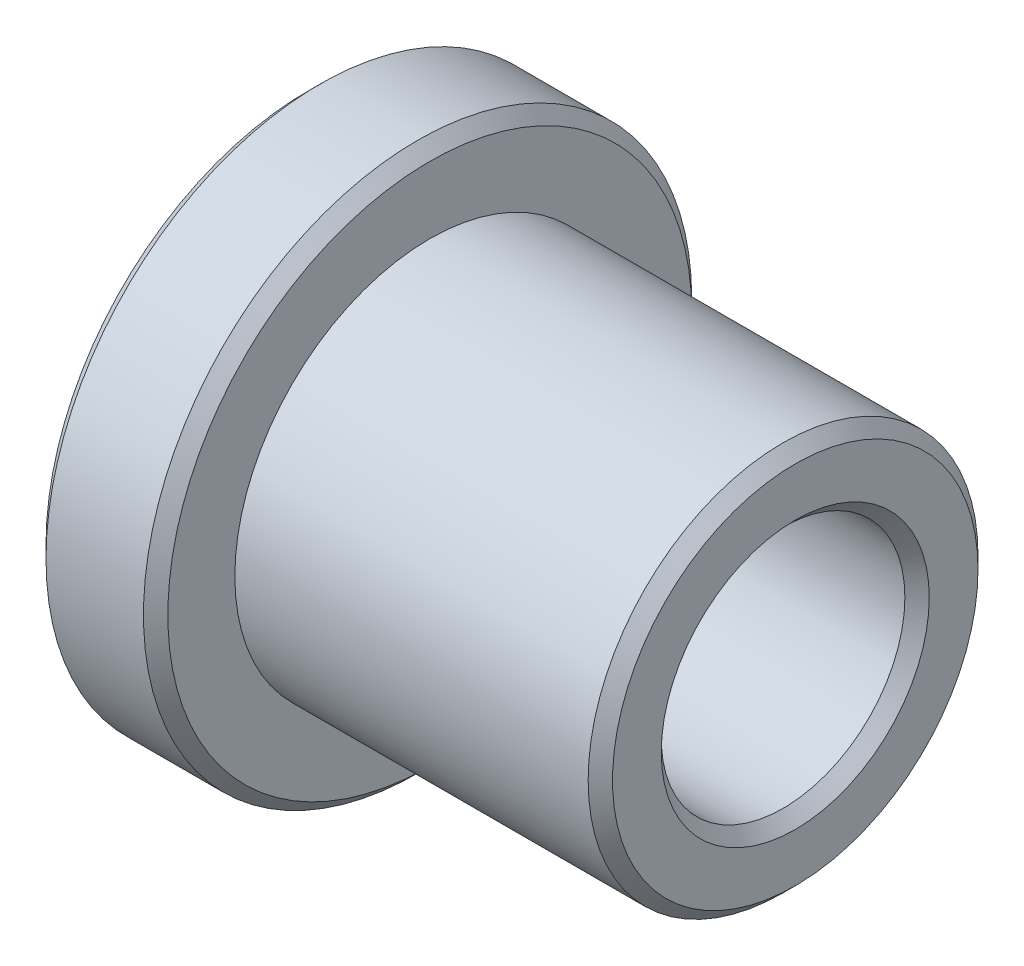
from build123d import *

# Parameters (mm, degrees)
CHAMFER1_SIZE = 1
CHAMFER2_SIZE = 3


with BuildPart() as part:
    # Sketch2 → Revolve1 (revolve)
    with BuildSketch(Plane.XY, mode=Mode.PRIVATE) as revolve1_sk:
        Polygon((0, 10), (0, 16), (-30, 16), (-30, 22.5), (-40, 22.5), (-40, 16), (-45, 16), (-45, 10), align=None)
    revolve(revolve1_sk.sketch.rotate(Axis((0, 0, 0), (-1, 0, 0)), 90), axis=Axis((0, 0, 0), (-1, 0, 0)))

    # Chamfer1
    chamfer1_edges = [part.edges().sort_by_distance(p)[0] for p in [
        (0, 0, 16),
        (-30, 0, 22.5),
        (-40, 0, 22.5),
        (-45, 0, 10),
        (0, 0, 10),
    ]]
    chamfer(chamfer1_edges, length=CHAMFER1_SIZE)

    # Chamfer2
    chamfer2_edges = [part.edges().sort_by_distance(p)[0] for p in [
        (-45, 0, 16),
    ]]
    chamfer(chamfer2_edges, length=CHAMFER2_SIZE)


solid = part.part
